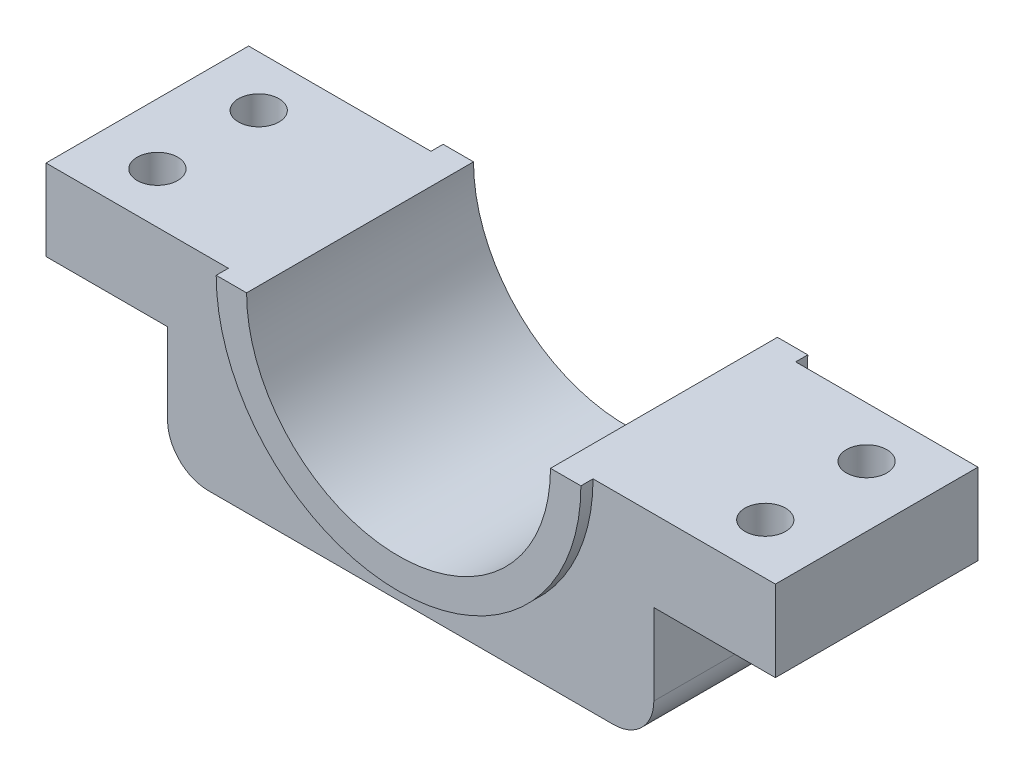
from build123d import *

# Parameters (mm, degrees)
SKETCH_1_W          = 120
SKETCH_1_H          = 50
EXTRUDE_1_DEPTH     = 50
SKETCH_2_R          = 37.5
CUT_EXTRUDE_1_DEPTH = 50
SKETCH_3_W          = 30
SKETCH_3_H          = 50
EXTRUDE_3_DEPTH     = 20
FILLET_1_R          = 10
SKETCH_5_R          = 5
CUT_EXTRUDE_2_DEPTH = 20
EXTRUDE_START       = 3
EXTRUDE_4_DEPTH     = 3


with BuildPart() as part:
    # 草图1 → 凸台-拉伸1 (new body)
    with BuildSketch(Plane(origin=(0, 0, 0), x_dir=(1, 0, 0), z_dir=(0, 1, 0))):
        Rectangle(SKETCH_1_W, SKETCH_1_H)
    extrude(amount=-EXTRUDE_1_DEPTH)

    # 草图2 → 切除-拉伸1 (cut)
    with BuildSketch(Plane.XY.offset(25)):
        Circle(SKETCH_2_R)
    extrude(amount=-CUT_EXTRUDE_1_DEPTH, mode=Mode.SUBTRACT)

    # 草图3 → 凸台-拉伸3 (add)
    with BuildSketch(Plane.XZ):
        with Locations((-75, 0)):
            Rectangle(SKETCH_3_W, SKETCH_3_H)
        with Locations((75, 0)):
            Rectangle(SKETCH_3_W, SKETCH_3_H)
    extrude(amount=EXTRUDE_3_DEPTH)

    # 圆角1
    fillet_1_edges = [part.edges().sort_by_distance(p)[0] for p in [
        (60, -50, 0),
        (-60, -50, 0),
    ]]
    fillet(fillet_1_edges, radius=FILLET_1_R)

    # 草图5 → 切除-拉伸2 (cut)
    with BuildSketch(Plane(origin=(0, 0, 0), x_dir=(1, 0, 0), z_dir=(0, 1, 0))):
        with Locations(Location((-75, 12.5, 0), (0, 0, 270))):
            Circle(SKETCH_5_R)
        with Locations(Location((-75, -12.5, 0), (0, 0, 270))):
            Circle(SKETCH_5_R)
        with Locations(Location((75, -12.5, 0), (0, 0, 90))):
            Circle(SKETCH_5_R)
        with Locations(Location((75, 12.5, 0), (0, 0, 90))):
            Circle(SKETCH_5_R)
    extrude(amount=-CUT_EXTRUDE_2_DEPTH, mode=Mode.SUBTRACT)

    # 草图6 → 凸台-拉伸4 (add)
    with BuildSketch(Plane.XY.offset(25).offset(EXTRUDE_START)):
        with BuildLine():
            Line((-45, 0), (-37.5, 0))
            ThreePointArc((-37.5, 0), (0, -37.5), (37.5, 0))
            Line((37.5, 0), (45, 0))
            ThreePointArc((45, 0), (0, -45), (-45, 0))
        make_face()
    extrude_4 = extrude(amount=-EXTRUDE_4_DEPTH)

    # 镜向1: 凸台-拉伸4 across plane
    add(extrude_4.mirror(Plane.XY))


solid = part.part
